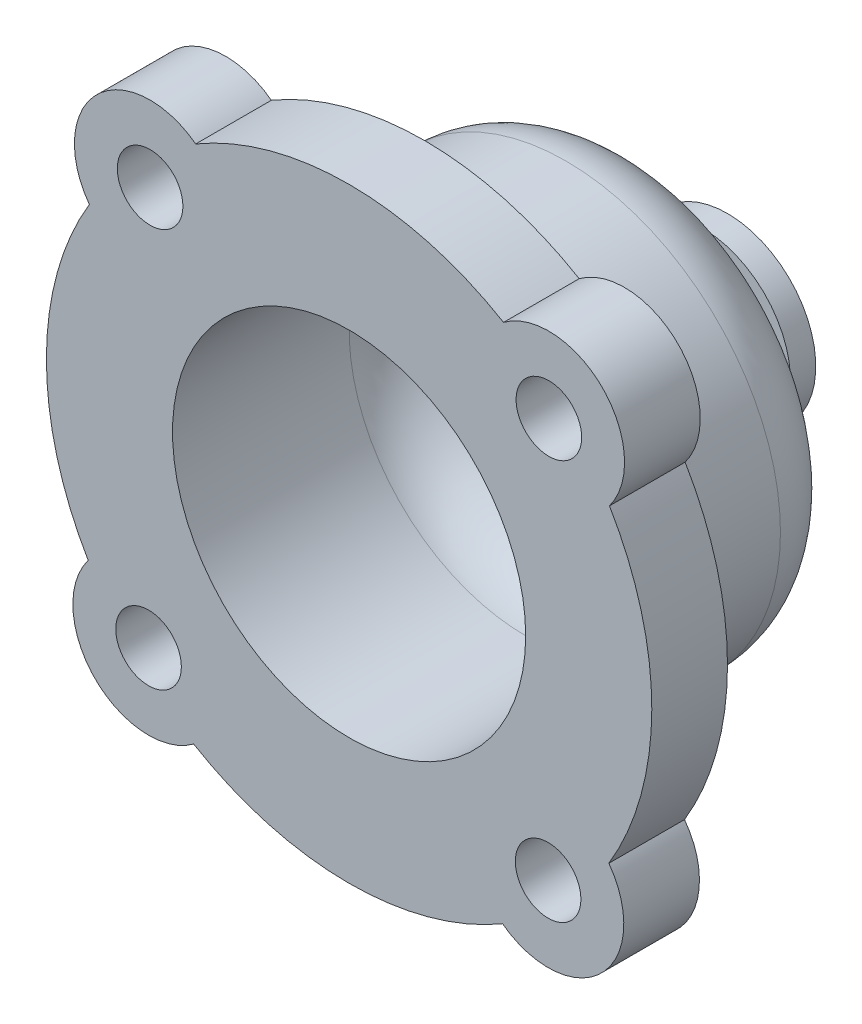
from build123d import *

# Parameters (mm, degrees)
SKETCH1_R           = 6.5
BOSS_EXTRUDE1_DEPTH = 15
CUT_EXTRUDE1_START  = -13
SKETCH2_R           = 13
CUT_EXTRUDE1_DEPTH  = 2
FILLET1_R           = 15
SKETCH4_R           = 27.5
BOSS_EXTRUDE2_DEPTH = 2
SKETCH5_R           = 7.25
CUT_EXTRUDE2_DEPTH  = 30
SKETCH6_R           = 35
CUT_EXTRUDE3_DEPTH  = 50
FILLET2_R           = 15


with BuildPart() as part:
    # Sketch1 → Boss-Extrude1 (new body)
    with BuildSketch(Plane.XY):
        with BuildLine():
            ThreePointArc((30.608172596, 51.605617624), (0.11519166, 59.999889424), (-30.409796101, 51.722763858))
            ThreePointArc((-30.409796101, 51.722763858), (-50.011440089, 50.39698265), (-51.487710544, 30.806097821))
            ThreePointArc((-51.487710544, 30.806097821), (-59.999557696, 0.230382895), (-51.722763858, -30.409796101))
            ThreePointArc((-51.722763858, -30.409796101), (-50.39698265, -50.011440089), (-30.806097821, -51.487710544))
            ThreePointArc((-30.806097821, -51.487710544), (-0.230382895, -59.999557696), (30.409796101, -51.722763858))
            ThreePointArc((30.409796101, -51.722763858), (50.011440089, -50.39698265), (51.487710544, -30.806097821))
            ThreePointArc((51.487710544, -30.806097821), (59.999889424, -0.11519166), (51.605617624, 30.608172596))
            ThreePointArc((51.605617624, 30.608172596), (50.204581464, 50.204581464), (30.608172596, 51.605617624))
        make_face()
        with Locations((39.597979746, 39.597979746)):
            Circle(SKETCH1_R, mode=Mode.SUBTRACT)
        with Locations((-39.445642887, 39.749732794)):
            Circle(SKETCH1_R, mode=Mode.SUBTRACT)
        with Locations((-39.749732794, -39.445642887)):
            Circle(SKETCH1_R, mode=Mode.SUBTRACT)
        with Locations((39.445642887, -39.749732794)):
            Circle(SKETCH1_R, mode=Mode.SUBTRACT)
    extrude(amount=BOSS_EXTRUDE1_DEPTH)

    # Sketch2 → Cut-Extrude1 (cut)
    with BuildSketch(Plane.XY.offset(15).offset(CUT_EXTRUDE1_START)):
        with Locations((-39.445642887, 39.749732794)):
            Circle(SKETCH2_R)
        with Locations((39.597979746, 39.597979746)):
            Circle(SKETCH2_R)
        with Locations((39.445642887, -39.749732794)):
            Circle(SKETCH2_R)
        with Locations((-39.749732794, -39.445642887)):
            Circle(SKETCH2_R)
    extrude(amount=-CUT_EXTRUDE1_DEPTH, mode=Mode.SUBTRACT)

    # Sketch3 → Revolve1 (revolve)
    with BuildSketch(Plane(origin=(0, 0, 0), x_dir=(1, 0, 0), z_dir=(0, 1, 0))):
        Polygon((-42.5, 0), (-42.5, 43), (-17.5, 43), (-17.5, 50), (-15, 50), (-15, 55), (-17.5, 55), (-17.5, 60), (0, 60), (0, 0), align=None)
    revolve(axis=Axis((0, 0, -60), (0, 0, 1)))

    # Fillet1
    fillet1_edges = [part.edges().sort_by_distance(p)[0] for p in [
        (42.5, 0, -43),
    ]]
    fillet(fillet1_edges, radius=FILLET1_R)

    # Sketch4 → Boss-Extrude2 (add)
    with BuildSketch(Plane(origin=(0, 0, -43), x_dir=(-1, 0, 0), z_dir=(0, 0, -1))):
        Circle(SKETCH4_R)
    extrude(amount=BOSS_EXTRUDE2_DEPTH)

    # Sketch5 → Cut-Extrude2 (cut)
    with BuildSketch(Plane(origin=(0, 0, -60), x_dir=(-1, 0, 0), z_dir=(0, 0, -1))):
        Circle(SKETCH5_R)
    extrude(amount=-CUT_EXTRUDE2_DEPTH, mode=Mode.SUBTRACT)

    # Sketch6 → Cut-Extrude3 (cut)
    with BuildSketch(Plane.XY.offset(15)):
        Circle(SKETCH6_R)
    extrude(amount=-CUT_EXTRUDE3_DEPTH, mode=Mode.SUBTRACT)

    # Fillet2
    fillet2_edges = [part.edges().sort_by_distance(p)[0] for p in [
        (-35, 0, -35),
    ]]
    fillet(fillet2_edges, radius=FILLET2_R)


solid = part.part
